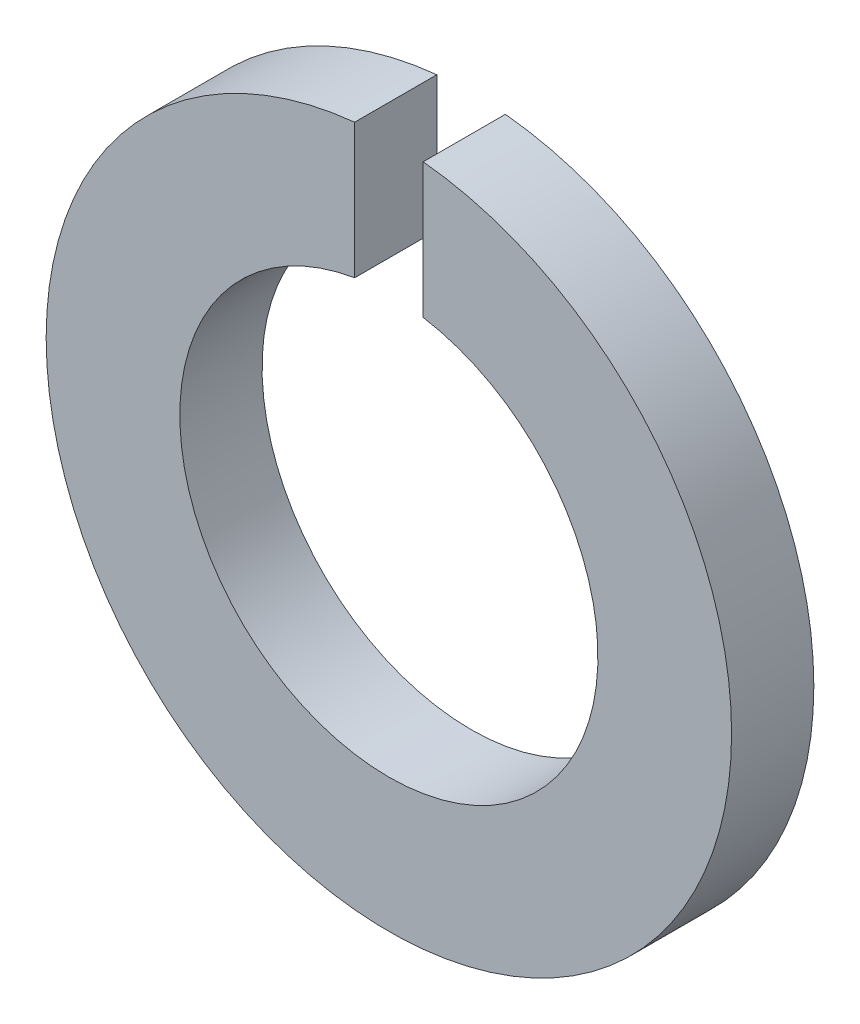
SolidWorks part; units mm, degrees
ref_plane "Front Plane" through (0, 0, 0) normal (0, 0, 1) x (1, 0, 0)
ref_plane "Top Plane" through (0, 0, 0) normal (0, 1, 0) x (1, 0, 0)
ref_plane "Right Plane" through (0, 0, 0) normal (1, 0, 0) x (0, 0, -1)
ref_plane "Plane4" through (0, 0, 229.8998) normal (0, 0, 1) x (1, 0, 0)
sketch "Sketch1" plane through (0, 0, 229.8998) normal (0, 0, 1) x (1, 0, 0)
  line L0 (0.5, 4.9749) -> (0.5, 3.0087)
  line L1 (-0.5, 3.0087) -> (-0.5, 4.9749)
  arc A0 (-0.5, 4.9749) -> (0.5, 4.9749) centre (0, 0) ccw
  arc A1 (0.5, 3.0087) -> (-0.5, 3.0087) centre (0, 0) cw
extrude "Boss-Extrude1" add sketch "Sketch1" against normal blind 1.2
